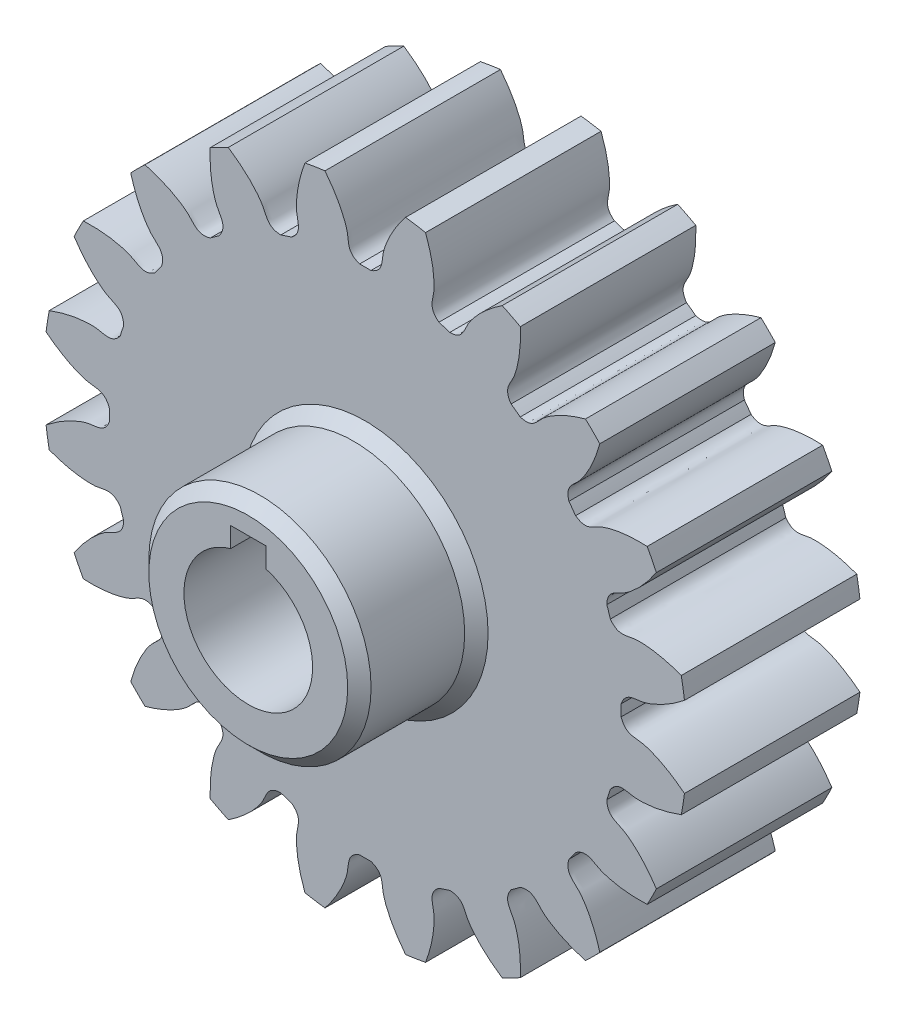
from build123d import *

# Parameters (mm, degrees)
SKETCH_1_R               = 55
EXTRUDE_1_DEPTH          = 30
CUT_EXTRUDE_1_DEPTH      = 84.366660003
PATTERN_CIRCULAR_1_COUNT = 20
CUT_EXTRUDE_2_DEPTH      = 83.795517166
EXTRUDE_START            = 20
SKETCH_5_R               = 19
EXTRUDE_2_DEPTH          = 20
CHAMFER_1_SIZE           = 2


with BuildPart() as part:
    # 草图1 → 凸台-拉伸1 (new body)
    with BuildSketch(Plane.XY):
        Circle(SKETCH_1_R)
    extrude(amount=EXTRUDE_1_DEPTH)

    # 草图2 → 切除-拉伸1 (cut, through all)
    with BuildSketch(Plane.XY):
        with BuildLine():
            ThreePointArc((0.966583002, 43.73932118), (0, 43.75), (-0.966583002, 43.73932118))
            add(Edge.make_bspline(
                [(-0.966583002, 43.73932118), (-3.055947024, 44.46737756), (-2.785420497, 45.935568494), (-3.064485282, 47.350047013), (-3.094460931, 47.48778307), (-3.131554449, 47.643173076), (-3.176460485, 47.81598418), (-3.229895701, 48.005957484), (-3.292560275, 48.21281414), (-3.365149357, 48.436253665), (-3.44834875, 48.675954735), (-3.542835499, 48.931575226), (-3.649276993, 49.202752503), (-3.768330511, 49.489103654), (-3.900642656, 49.790225757), (-4.046848823, 50.105696157), (-4.207572667, 50.435072754), (-4.383425584, 50.777894307), (-4.575006192, 51.133680749), (-4.782899828, 51.50193352), (-5.007678047, 51.882135904), (-5.249898131, 52.273753389), (-5.510102607, 52.676234027), (-5.788818779, 53.089008819), (-6.086558255, 53.511492101), (-6.403816503, 53.943081952), (-6.741072402, 54.383160603), (-7.098787808, 54.831094863), (-7.477407132, 55.286236557), (-7.877356926, 55.747922972), (-8.299045483, 56.215477314), (-8.742862444, 56.688209175), (-9.209178422, 57.165415012), (-9.698344631, 57.646378634), (-10.210692532, 58.130371697), (-10.746533492, 58.616654211), (-11.306158447, 59.104475055), (-11.889837592, 59.593072497), (-12.497820059, 60.08167473), (-13.130333672, 60.569500408), (-13.787584497, 61.0557592), (-14.707367954, 61.708199338), (-15.419662063, 62.181663005), (-15.905789909, 62.491259298)],
                knots=[0, 0, 0, 0, 0.165916003, 0.170905922, 0.176663519, 0.183188797, 0.190481754, 0.198542391, 0.207370708, 0.216966704, 0.22733038, 0.238461736, 0.250360771, 0.263027487, 0.276461881, 0.290663956, 0.30563371, 0.321371144, 0.337876258, 0.355149051, 0.373189524, 0.391997677, 0.411573509, 0.431917021, 0.453028213, 0.474907084, 0.497553636, 0.520967867, 0.545149777, 0.570099367, 0.595816637, 0.622301587, 0.649554216, 0.677574526, 0.706362514, 0.735918183, 0.766241531, 0.797332559, 0.829191267, 0.861817654, 0.895211721, 0.929373468, 1, 1, 1, 1], degree=3))
            ThreePointArc((-15.905789909, 62.491259298), (0, 64.483731602), (15.905789909, 62.491259298))
            add(Edge.make_bspline(
                [(0.966583002, 43.73932118), (3.055947024, 44.46737756), (2.785420497, 45.935568494), (3.064485282, 47.350047013), (3.094460931, 47.48778307), (3.131554449, 47.643173076), (3.176460485, 47.81598418), (3.229895701, 48.005957484), (3.292560275, 48.21281414), (3.365149357, 48.436253665), (3.44834875, 48.675954735), (3.542835499, 48.931575226), (3.649276993, 49.202752503), (3.768330511, 49.489103654), (3.900642656, 49.790225757), (4.046848823, 50.105696157), (4.207572667, 50.435072754), (4.383425584, 50.777894307), (4.575006192, 51.133680749), (4.782899828, 51.50193352), (5.007678047, 51.882135904), (5.249898131, 52.273753389), (5.510102607, 52.676234027), (5.788818779, 53.089008819), (6.086558255, 53.511492101), (6.403816503, 53.943081952), (6.741072402, 54.383160603), (7.098787808, 54.831094863), (7.477407132, 55.286236557), (7.877356926, 55.747922972), (8.299045483, 56.215477314), (8.742862444, 56.688209175), (9.209178422, 57.165415012), (9.698344631, 57.646378634), (10.210692532, 58.130371697), (10.746533492, 58.616654211), (11.306158447, 59.104475055), (11.889837592, 59.593072497), (12.497820059, 60.08167473), (13.130333672, 60.569500408), (13.787584497, 61.0557592), (14.707367954, 61.708199338), (15.419662063, 62.181663005), (15.905789909, 62.491259298)],
                knots=[0, 0, 0, 0, 0.165916003, 0.170905922, 0.176663519, 0.183188797, 0.190481754, 0.198542391, 0.207370708, 0.216966704, 0.22733038, 0.238461736, 0.250360771, 0.263027487, 0.276461881, 0.290663956, 0.30563371, 0.321371144, 0.337876258, 0.355149051, 0.373189524, 0.391997677, 0.411573509, 0.431917021, 0.453028213, 0.474907084, 0.497553636, 0.520967867, 0.545149777, 0.570099367, 0.595816637, 0.622301587, 0.649554216, 0.677574526, 0.706362514, 0.735918183, 0.766241531, 0.797332559, 0.829191267, 0.861817654, 0.895211721, 0.929373468, 1, 1, 1, 1], degree=3))
        make_face()
    cut_extrude_1 = extrude(amount=CUT_EXTRUDE_1_DEPTH, mode=Mode.SUBTRACT)

    # 阵列(圆周)1: 切除-拉伸1 ×20 about axis
    pattern_circular_1_axis = Axis((0, 0, -1.5), (0, 0, 1))
    for i in range(1, PATTERN_CIRCULAR_1_COUNT):
        add(cut_extrude_1.rotate(pattern_circular_1_axis, i * 360 / PATTERN_CIRCULAR_1_COUNT), mode=Mode.SUBTRACT)

    # 草图4 → 切除-拉伸2 (cut, through all)
    with BuildSketch(Plane.XY.offset(30)):
        with BuildLine():
            ThreePointArc((3, 10.583005244), (0, 11), (-3, 10.583005244))
            Line((-3, 10.583005244), (-3, 8))
            Line((-3, 8), (3, 8))
            Line((3, 8), (3, 10.583005244))
        make_face()
        with BuildLine():
            Line((-3, 8), (-3, 10.583005244))
            ThreePointArc((-3, 10.583005244), (-6.633249581, -8.774964387), (11, 0))
            ThreePointArc((11, 0), (8.774964387, 6.633249581), (3, 10.583005244))
            Line((3, 10.583005244), (3, 8))
            Line((3, 8), (-3, 8))
        make_face()
        with BuildLine():
            ThreePointArc((3, 10.583005244), (0, 11), (-3, 10.583005244))
            Line((-3, 10.583005244), (-3, 8))
            Line((-3, 8), (3, 8))
            Line((3, 8), (3, 10.583005244))
        make_face()
        with BuildLine():
            Line((-3, 8), (-3, 10.583005244))
            ThreePointArc((-3, 10.583005244), (-6.633249581, -8.774964387), (11, 0))
            ThreePointArc((11, 0), (8.774964387, 6.633249581), (3, 10.583005244))
            Line((3, 10.583005244), (3, 8))
            Line((3, 8), (-3, 8))
        make_face()
        with BuildLine():
            Line((3, 14), (-3, 14))
            Line((-3, 14), (-3, 10.583005244))
            ThreePointArc((-3, 10.583005244), (0, 11), (3, 10.583005244))
            Line((3, 10.583005244), (3, 14))
        make_face()
    extrude(amount=-CUT_EXTRUDE_2_DEPTH, mode=Mode.SUBTRACT)

    # 草图5 → 凸台-拉伸2 (add)
    with BuildSketch(Plane.XY.offset(30).offset(EXTRUDE_START)):
        Circle(SKETCH_5_R)
        with BuildLine():
            Line((-3, 14), (-3, 10.583005244))
            ThreePointArc((-3, 10.583005244), (0, -11), (3, 10.583005244))
            Line((3, 10.583005244), (3, 14))
            Line((3, 14), (-3, 14))
        make_face(mode=Mode.SUBTRACT)
    extrude(amount=-EXTRUDE_2_DEPTH)

    # 倒角1
    chamfer_1_edges = [part.edges().sort_by_distance(p)[0] for p in [
        (-19, 0, 50),
        (-19, 0, 30),
    ]]
    chamfer(chamfer_1_edges, length=CHAMFER_1_SIZE)


solid = part.part
